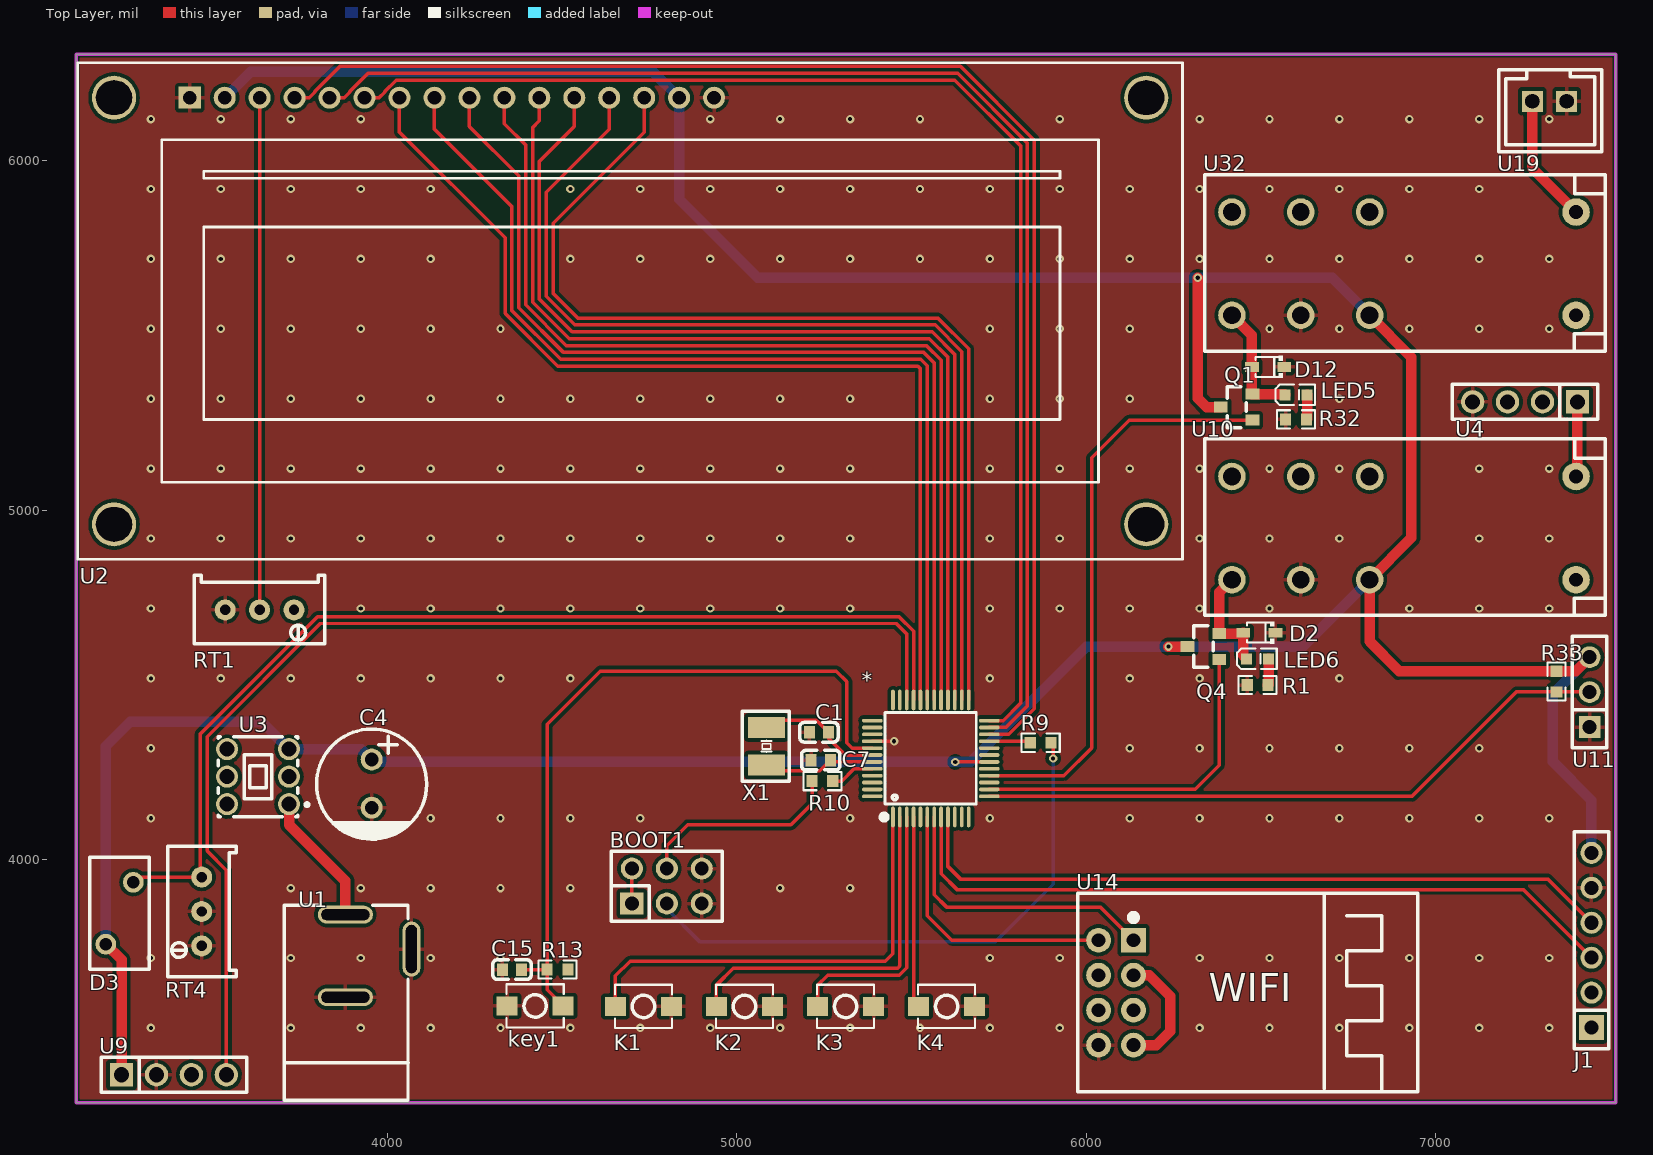
[diagram p0: Top Layer view]
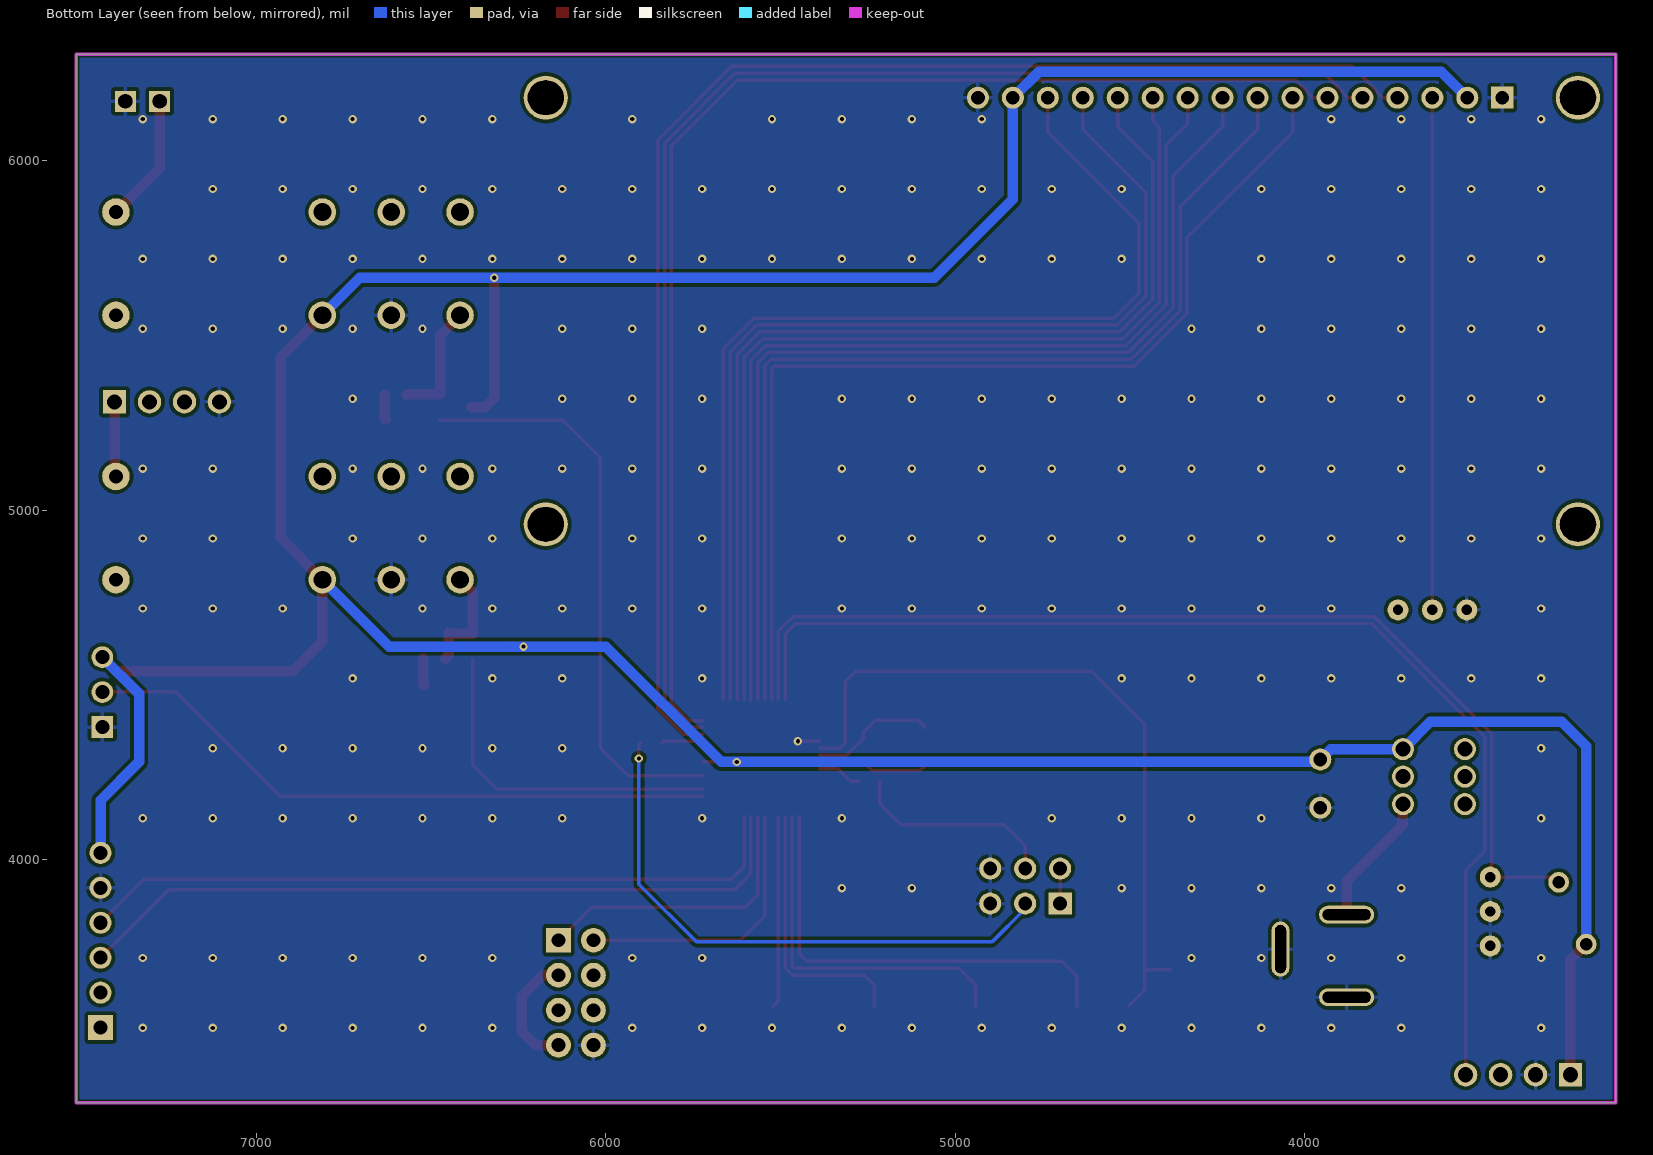
[diagram p1: Bottom Layer view, seen from below]
# Altium PCB MISC51945.pcbdoc
Units mil, origin at the board's own origin, x right, y up, seen from the top; angles counter-clockwise.
Board outline 4405 x 3000 mil, 2 copper layers (Top Layer, Bottom Layer), stack 62.206 mil thick; 38 components, 51 nets, 180 pads, 213 vias.

## Layer stack, top to bottom
Top Solder Mask Layer: solder mask 0.394, Dk 3.3
Top Layer: signal copper 1.379
Dielectric1: surface 59.449, FR4, Dk 4.5
Bottom Layer: signal copper 1.378
Bottom Solder Mask Layer: solder mask 0.394, Dk 3.3

## Board outline
3110,6305 3110,3305 7515,3305 7515,6305

## Design rules (kind name [scope] priority, off if disabled: settings)
BoardOutlineClearance copperThickness2oz_1 [All] p2 off: genericclearance=7.99 ignorepadtopadclearanceinfootprint=FALSE except(0: Arc-SplitContinuation Track-SplitContinuation SMDPad-SplitContinuation THPad-SplitContinuation Via-SplitContinuation Fill-SplitContinuation Region-SplitContinuation Poly-SplitContinuation Text-SplitContinuation Hole-SplitContinuation; 5.98: Arc-CutoutEdge SMDPad-CutoutEdge THPad-CutoutEdge Via-CutoutEdge Fill-CutoutEdge Region-CutoutEdge Text-CutoutEdge; 6.93: Hole-OutlineEdge Hole-CutoutEdge; 10: Poly-OutlineEdge Poly-CutoutEdge; 11.81: Arc-OutlineEdge Track-OutlineEdge SMDPad-OutlineEdge THPad-OutlineEdge Via-OutlineEdge Fill-OutlineEdge Region-OutlineEdge Text-OutlineEdge Track-CutoutEdge)
BoardOutlineClearance copperThickness1oz_1 [All] p4: genericclearance=4.02 ignorepadtopadclearanceinfootprint=FALSE except(0: Arc-SplitContinuation Track-SplitContinuation SMDPad-SplitContinuation THPad-SplitContinuation Via-SplitContinuation Fill-SplitContinuation Region-SplitContinuation Poly-SplitContinuation Text-SplitContinuation Hole-SplitContinuation; 6: SMDPad-CutoutEdge THPad-CutoutEdge Via-CutoutEdge Fill-CutoutEdge Region-CutoutEdge Text-CutoutEdge; 6.93: Hole-OutlineEdge Hole-CutoutEdge; 10: Poly-OutlineEdge Poly-CutoutEdge; 11.8: Arc-OutlineEdge Track-OutlineEdge SMDPad-OutlineEdge THPad-OutlineEdge Via-OutlineEdge Fill-OutlineEdge Region-OutlineEdge Text-OutlineEdge; 11.81: Arc-CutoutEdge Track-CutoutEdge)
Clearance copperThickness2oz [All] p1 off: gap=7.99 ignorepadtopadclearanceinfootprint=FALSE except(5.98: SMDPad-Track SMDPad-SMDPad THPad-Track SMDPad-THPad THPad-THPad Track-Via SMDPad-Via THPad-Via Via-Via Fill-Track Region-Track Fill-SMDPad Region-SMDPad Fill-THPad Region-THPad Fill-Via Region-Via Fill-Fill Fill-Region Region-Region Arc-Track Arc-SMDPad Arc-THPad Arc-Via Fill-Arc Region-Arc Arc-Arc Text-Track SMDPad-Text Text-THPad Text-Via Fill-Text Region-Text Arc-Text Text-Text; 6.93: Hole-Track Hole-SMDPad Hole-THPad Hole-Via Fill-Hole Region-Hole Hole-Arc Hole-Text; 10: Poly-Track Poly-SMDPad Poly-THPad Poly-Via Poly-Fill Poly-Region Poly-Poly Poly-Arc Poly-Text Poly-Hole)
Clearance copperThickness1oz [All] p3: gap=4.02 ignorepadtopadclearanceinfootprint=FALSE except(5.98: SMDPad-Track SMDPad-SMDPad THPad-Track SMDPad-THPad THPad-THPad Track-Via SMDPad-Via THPad-Via Via-Via Fill-Track Region-Track Fill-SMDPad Region-SMDPad Fill-THPad Region-THPad Fill-Via Region-Via Fill-Fill Fill-Region Region-Region; 6: Arc-Track Arc-SMDPad Arc-THPad Arc-Via Fill-Arc Region-Arc Arc-Arc Text-Track SMDPad-Text Text-THPad Text-Via Fill-Text Region-Text Arc-Text Text-Text; 6.93: Hole-Track Hole-SMDPad Hole-THPad Hole-Via Fill-Hole Region-Hole Hole-Arc Hole-Text; 10: Poly-Track Poly-SMDPad Poly-THPad Poly-Via Poly-Fill Poly-Region Poly-Poly Poly-Arc Poly-Text Poly-Hole)
DiffPairsRouting differentialPair [All] p1: maxlimit=6 minlimit=6 mostfreqgap=6 toplayer_minwidth=5 toplayer_prefwidth=10 toplayer_maxwidth=100 toplayer_mingap=6 toplayer_prefgap=6 toplayer_maxgap=6 bottomlayer_minwidth=5 bottomlayer_prefwidth=10 bottomlayer_maxwidth=100 bottomlayer_mingap=6 bottomlayer_prefgap=6 bottomlayer_maxgap=6 maxuncoupledlength=10
HoleToHoleClearance otherClearance [All] p1: gap=11.81 allowstackedmicrovias=TRUE
Length netLength [All] p1: minlimit=0 maxlimit=0
MatchedLengths netLengthTolerance [All] p1: tolerance=1000
PasteMaskExpansion pasteMaskExpansion [All] p1: expansion=0
PlaneConnect innerPlane [All] p1: planeconnectstyle=Relief reliefexpansion=20 reliefentries=4 reliefconductorwidth=10 reliefairgap=10
PolygonConnect copperRegion [(InNet('GND'))] p1: connectstyle=Relief reliefconductorwidth=10 reliefentries=4 polygonreliefangle="90 Angle" airgapwidth=10 via.connectstyle=Relief via.reliefconductorwidth=10 via.reliefentries=4 via.polygonreliefangle="90 Angle" via.airgapwidth=10
RoutingVias viaSize [All] p1: holewidth=12.01 width=24.02 viastyle="Through Hole" minholewidth=11.81 minwidth=19.68 maxholewidth=248.03 maxwidth=393.7
SolderMaskExpansion solderMaskExpansion [IsVia] p1: expansion=-1000 istentingtop=TRUE
SolderMaskExpansion solderMaskExpansion [All] p2: expansion=2 istentingtop=FALSE
Width copperThickness2oz_2 [All] p1 off: maxlimit=100 minlimit=8 preferedwidth=10
Width copperThickness1oz_2 [All] p2: maxlimit=100 minlimit=5 preferedwidth=10

## Components (designator, comment, footprint, x,y, rotation, side; value= is the part's Value field where it differs from the comment)
* "程序下载口" LQFP-48_L7.0-W7.0-P0.50-LS9.0-BL 5555,4290 r0 top
BOOT1 "Header 3X2" HDR-TH_6P-P2.54-V-F-R2-C3-S2.54 4800,3925 r0 top
C1 "20pF" C0603 5235,4365 r0 top
C4 "1000UF" CAP-TH_BD8.0-P3.50-D0.6-FD_1 3955.58,4218 r270 top
C7 "20pF" C0603 5240,4285 r0 top
C15 "104" C0603 4357.19,3686.05 r0 top
D2 "IN4148" SOD-323_L1.8-W1.3-LS2.5-RD 6495,4650 r180 top
D3 "光敏电阻" RES-TH_L8.0-W4.4-P4.50-D0.6-S2.0 3234.3,3847.2 r90 top
D12 "IN4148" SOD-323_L1.8-W1.3-LS2.5-RD 6520,5410 r180 top
J1 "" HDR-TH_6P-P2.54-V-F 7445,3770 r90 top
K1 "" Key_SMD_3x4x2 4733,3580.6 r180 top
K2 "" Key_SMD_3x4x2 5022.12,3580.6 r180 top
K3 "" Key_SMD_3x4x2 5311.24,3580.6 r180 top
K4 "" Key_SMD_3x4x2 5600.36,3580.6 r180 top
key1 "KEY_M" Key_SMD_3x4x2 4423.29,3582.1 r180 top
LED5 "LED" LED0603 6600,5330 r0 top
LED6 "LED" LED0603 6490,4575 r0 top
Q1 "S8050" S8050_SOT-23 6430,5295 r0 top
Q4 "S8050" S8050_SOT-23 6335,4610 r0 top
R1 "1K" R0603 6490,4500 r0 top
R9 "10K" R0603 5869.32,4335 r0 top
R10 "10K" R0603 5245,4225 r0 top
R13 "10 K" R0603 4487.19,3686.05 r180 top
R32 "1K" R0603 6600,5260 r0 top
R33 "10K" R0603 7344.9,4509.9 r90 top
RT1 "10K" R_3296 3635,4710 r180 top
RT4 "10K" R_3296 3464.3,3852.2 r90 top
U1 "POW" DC-2.0 3870,3720 r270 top
U2 "LCD1602" LCD1602 4695,5570 r0 top
U3 "SWITCH" SW-TH_6P-L5.8-W5.8-P2.00-LS4.5-TR 3630.58,4238 r270 top
U4 "" HDR-TH_4P-P2.54-V-F 7255,5310 r180 top
U9 "" HDR-TH_4P-P2.54-V-F 3390,3385 r0 top
U10 "JDQ-5" RELAY-TH_FTR-K1CK024W 6908.81,4948.98 r0 top
U11 "DHT11" HDR-TH_3P-P2.54-V-F 7439.9,4479.9 r90 top
U14 "ESP8266" WIFIM-TH_8P-L24.7-W14.4-P2.54 6085,3620 r0 top
U19 "" CONN-TH_XH2.54-2P 7325,6170 r180 top
U32 "JDQ-5" RELAY-TH_FTR-K1CK024W 6908.81,5705.51 r0 top
X1 "8MHz" CRYSTAL-SMD_L3.2-W2.5_3225-8MHZ 5085.08,4324.89 r90 top

## Footprints (in the part's own frame and the unit in brackets; to place one, negate y for a bottom-side part, rotate by r counter-clockwise, add the part's x,y. Pads: shape width x height; smd on the part's side, far side on the other; paste and mask are expansions set on the pad)
C0603 [mm]
  rect 0.8x0.9 smd: 1(-0.7,0) 2(0.7,0)
  silkscreen extent -1.39,-0.71 1.39,0.71
CAP-TH_BD8.0-P3.50-D0.6-FD_1 [mm]
  round 1.6 hole 1: 1(-1.75,0) 2(1.75,0)
  silkscreen extent -3.96,-4 4.04,4
CONN-TH_XH2.54-2P [mil]
  rect 60x60 hole 39.37 slot 41.34 at 0 deg paste+0 mask+1.97: 1(-49.22,0) 2(49.21,0)
  silkscreen extent -150,-90 145,145
CRYSTAL-SMD_L3.2-W2.5_3225-8MHZ [mil]
  rect 60x106.3 smd paste+0 mask+1.97: 1(-53.62,0) 2(53.62,0)
  silkscreen extent -100,-65 100,70
DC-2.0 [mil]
  oval 157.5x51.2 hole 31.5 slot 137.8 at 0 deg paste+0 mask+2: 2(-24.7,199.5)
  oval 51.2x157.5 hole 31.5 slot 137.8 at 90 deg paste+0 mask+2: 3(113.1,10.5) 4(-123.1,10.5)
  silkscreen extent -151,-165 408,190
HDR-TH_3P-P2.54-V-F [mil]
  rect 62x62 hole 40.16: 1(-100,0)
  round 62 hole 40.16: 2(0,0) 3(100,0)
  silkscreen extent -160,-49 160,49
HDR-TH_4P-P2.54-V-F [mm]
  rect 1.7x1.7 hole 1.1: 1(-3.81,0)
  round 1.7 hole 1.1: 2(-1.27,0) 3(1.27,0) 4(3.81,0)
  silkscreen extent -5.29,-1.27 5.29,1.27
HDR-TH_6P-P2.54-V-F [mm]
  rect 1.8x1.8 hole 1.02: 1(-6.35,0)
  round 1.6 hole 1.02: 2(-3.81,0) 3(-1.27,0) 4(1.27,0) 5(3.81,0) 6(6.35,0)
  silkscreen extent -7.87,-1.25 7.87,1.25
HDR-TH_6P-P2.54-V-F-R2-C3-S2.54 [mm]
  rect 1.7x1.6 hole 1: 1(-2.54,-1.27)
  round 1.6 hole 1: 2(-2.54,1.27) 3(0,-1.27) 4(0,1.27) 5(2.54,-1.27) 6(2.54,1.27)
  silkscreen extent -4.04,-2.54 4.04,2.54
Key_SMD_3x4x2 [mm]
  rect 1.53x1.36 smd paste+0 mask+0.051: 1(-2.035,0) 2(2.035,0)
  silkscreen extent -2.08,-1.58 2.08,1.58
LCD1602 [mm]
  round 3.2 hole 2.5 slot 2.625 at 0 deg: 0(-37.5,-15.5) 0(-37.5,15.5) 0(37.5,-15.5) 0(37.5,15.5)
  rect 1.6x1.6 hole 1: 1(-32,15.5)
  round 1.6 hole 1: 2(-29.46,15.5) 3(-26.92,15.5) 4(-24.38,15.5) 5(-21.84,15.5) 6(-19.3,15.5) 7(-16.76,15.5) 8(-14.22,15.5) 9(-11.68,15.5) 10(-9.14,15.5) 11(-6.6,15.5) 12(-4.06,15.5) 13(-1.52,15.5) 14(1.02,15.5) 15(3.56,15.5) 16(6.1,15.5)
  silkscreen extent -40.13,-18.03 40.13,18.03
LED0603 [mm]
  rect 0.8x0.8 smd: 1(-0.799,-0.003) 2(0.799,0.003)
  silkscreen extent -1.49,-0.75 1.39,0.76
LQFP-48_L7.0-W7.0-P0.50-LS9.0-BL [mm]
  oval 0.27x1.5 smd paste+0 mask+0.05: 1(-2.75,-4.25) 2(-2.25,-4.25) 3(-1.75,-4.25) 4(-1.25,-4.25) 5(-0.75,-4.25) 6(-0.25,-4.25) 7(0.25,-4.25) 8(0.75,-4.25) 9(1.25,-4.25) 10(1.75,-4.25) 11(2.25,-4.25) 12(2.75,-4.25) 25(2.75,4.25) 26(2.25,4.25) 27(1.75,4.25) 28(1.25,4.25) 29(0.75,4.25) 30(0.25,4.25) 31(-0.25,4.25) 32(-0.75,4.25) 33(-1.25,4.25) 34(-1.75,4.25) 35(-2.25,4.25) 36(-2.75,4.25)
  oval 1.5x0.27 smd paste+0 mask+0.05: 13(4.25,-2.75) 14(4.25,-2.25) 15(4.25,-1.75) 16(4.25,-1.25) 17(4.25,-0.75) 18(4.25,-0.25) 19(4.25,0.25) 20(4.25,0.75) 21(4.25,1.25) 22(4.25,1.75) 23(4.25,2.25) 24(4.25,2.75) 37(-4.25,2.75) 38(-4.25,2.25) 39(-4.25,1.75) 40(-4.25,1.25) 41(-4.25,0.75) 42(-4.25,0.25) 43(-4.25,-0.25) 44(-4.25,-0.75) 45(-4.25,-1.25) 46(-4.25,-1.75) 47(-4.25,-2.25) 48(-4.25,-2.75)
  silkscreen extent -3.59,-4.46 3.3,3.34
R0603 [mil]
  rect 31.75x34.02 smd paste-3937.01 mask+2: 1(-29.66,0) 2(29.66,0)
  silkscreen extent -55,-26 55,26
R_3296 [mil]
  round 60 hole 30 paste+0 mask+2: 1(-98.4,-5) 2(0,-5) 3(98.4,-5)
  silkscreen extent -187,-103 187,92
RELAY-TH_FTR-K1CK024W [mm]
  round 2 hole 1.3: 1(-12.5,-3.75) 2(-7.5,-3.75) 3(-2.5,-3.75) 6(-2.5,3.75) 7(-7.5,3.75) 8(-12.5,3.75)
  round 2 hole 1: 4(12.5,-3.75) 5(12.5,3.75)
  silkscreen extent -14.48,-6.35 14.6,6.48
RES-TH_L8.0-W4.4-P4.50-D0.6-S2.0 [mm]
  round 1.5 hole 0.9 paste+0 mask+0.05: 1(-2.25,1) 2(2.25,-1)
  silkscreen extent -4.06,-2.16 4.06,2.16
S8050_SOT-23 [mm]
  rect 1x0.8 smd paste+0 mask+0.051: 1(1.15,-0.95) 2(1.15,0.95) 3(-1.15,0)
  silkscreen extent -0.7,-1.5 0.7,1.5
SOD-323_L1.8-W1.3-LS2.5-RD [mm]
  rect 1x0.7 smd: 1(-1.172,0) 2(1.172,0)
  silkscreen extent -1.08,-0.8 0.9,0.8
SW-TH_6P-L5.8-W5.8-P2.00-LS4.5-TR [mm]
  round 1.6 hole 1.1: 1(2,2.25) 2(0,2.25) 3(-2,2.25) 4(-2,-2.25) 5(0,-2.25) 6(2,-2.25)
  silkscreen extent -2.9,-2.9 2.9,3.68
WIFIM-TH_8P-L24.7-W14.4-P2.54 [mm]
  rect 1.8x1.8 hole 1 paste+0 mask+0.05: 1(1.27,3.81)
  round 1.8 hole 1 paste+0 mask+0.05: 2(1.27,1.27) 3(1.27,-1.27) 4(1.27,-3.81) 5(-1.27,3.81) 6(-1.27,1.27) 7(-1.27,-1.27) 8(-1.27,-3.81)
  silkscreen extent -2.77,-7.19 21.93,7.24

## Via types
v1: diameter 24.02, hole 12, Top Layer to Bottom Layer, 213 vias

## Nets (pads, with @x,y where several pads share a name; then routed paths per layer and width w, separated by ;. In a path a pad name is that pad's centre, name@x,y a point inside that pad or via, vN(x,y) a via of type N, cw(c..) or ccw(c..) an arc to the next point about the centre after c; other vN are vias at no path point)
3.3V: R13.1
$2N44: *.20
$2N45: *.26 U2.13 | length 2893.2
  Top Layer w10: U2.13 4635.16,6089.82 4455.31,5909.97 4455.31,5611.84 4536.97,5530.18 5567.32,5530.18 5643.58,5453.92 *.26
$2N46: *.27 U2.12 | length 2859.9
  Top Layer w10: U2.12 4535.16,6097.97 4435.63,5998.44 4435.63,5603.69 4528.82,5510.5 5559.17,5510.5 5623.9,5445.77 *.27
$2N47: *.29 U2.10 | length 2844
  Top Layer w10: U2.10 4335.16,6106.13 4396.26,6045.03 4396.26,5587.38 4512.51,5471.13 5542.86,5471.13 5584.53,5429.46 *.29
$2N48: *.30 U2.9 | length 2877.3
  Top Layer w10: U2.9 4235.16,6097.97 4376.57,5956.56 4376.57,5579.23 4504.36,5451.44 5534.71,5451.44 5564.84,5421.31 *.30
$2N49: *.31 U2.8 | length 2910.5
  Top Layer w10: U2.8 4135.16,6089.82 4356.89,5868.09 4356.89,5571.08 4496.21,5431.76 5526.55,5431.76 5545.16,5413.16 *.31
$2N50: *.32 U2.7 | length 2943.8
  Top Layer w10: U2.7 4035.16,6081.67 4337.2,5779.63 4337.2,5562.92 4488.05,5412.07 5518.4,5412.07 5525.47,5405 *.32
$2N51: *.28 U2.11 | length 2826.6
  Top Layer w10: U2.11 4435.16,6114.28 4415.94,6095.06 4415.94,5595.54 4520.67,5490.81 5551.01,5490.81 5604.21,5437.62 *.28
$2N52: RT1.2 U2.3 | length 1465.3
  Top Layer w10: RT1.2 3635,6180.08 U2.3
$2N54: BOOT1.3 R9.2 | length 1635.2
  Top Layer w10: R9.2 5905,4328.98 v1(5905,4290)
  Bottom Layer w10: BOOT1.3 4800,3860 4895,3765 5740,3765 5905,3930 v1(5905,4290)
$2N55: BOOT1.4 R10.1 | length 594.8
  Top Layer w10: BOOT1.4 4800,4040 4860,4100 5155,4100 5215.34,4160.34 R10.1
$2N56: *.41 C15.2 key1.1 R13.2 | length 2084.4
  Top Layer w10: C15.2 R13.2 ; key1.1 4457.53,3627.97 R13.2 ; *.41 5330.47,4319.53 5315,4335 5315,4510 5285,4540 4610,4540 4457.53,4387.53 R13.2
$2N57: *.42 C1.2 X1.2 | length 363.3
  Top Layer w10: X1.2 5106.57,4400 5227.56,4400 C1.2 5262.56,4347.44 5310.16,4299.84 *.42
$2N58: U1.4 U3.1 | length 383
  Top Layer w30: U3.1 3719.16,4100.84 3880.5,3939.5 U1.4
$2N59: *.19
$2N60: D2.2 LED6.1 Q4.2 U10.1 | length 317.8
  Top Layer w30: U10.1 6380.28,4764.93 Q4.2 6446.24,4647.4 D2.2 6448.84,4584.55 LED6.1
$2N61: U19.2 U32.5 | length 368.7
  Top Layer w30: U19.2 7275.78,5978.3 U32.5
$2N62: D12.2 LED5.1 Q1.2 U32.1 | length 344
  Top Layer w30: U32.1 6473.84,5500.73 D12.2 6473.84,5333.84 Q1.2 6565.99,5332.4 LED5.1
$2N63: *.10
$2N64: *.25 U2.14 | length 2926.4
  Top Layer w10: U2.14 4735.16,6081.67 4475,5821.51 4475,5620 4545.13,5549.87 5575.48,5549.87 5663.27,5462.08 *.25
$2N65: *.24 U2.6 | length 3680.8
  Top Layer w10: U2.6 3976.66,6180.24 3992.68,6196.26 3992.68,6197.84 4025.47,6230.63 5623.69,6230.63 5811.79,6042.53 5811.79,4448.21 5761.85,4398.27 *.24
$2N66: *.23 U2.5 | length 3854.2
  Top Layer w10: U2.5 3876.66,6180.24 3892.68,6196.26 3892.68,6197.84 3945.16,6250.32 5631.85,6250.32 5831.48,6050.69 5831.48,4440.06 5770,4378.58 *.23
$2N67: *.22 U2.4 | length 4027.6
  Top Layer w10: U2.4 3776.66,6180.24 3792.68,6196.26 3792.68,6197.84 3864.84,6270 5640,6270 5851.16,6058.84 5851.16,4431.9 5778.16,4358.9 *.22
$2N69: *.5
$2N70: *.11
$2N71: *.12
$2N72: U4.1 U10.5 | length 215.1
  Top Layer w30: U10.5 7405,5100.68 U4.1
$2N73: *.15
$2N76: *.8 J1.3 | length 2122.3
  Top Layer w10: *.8 5584.53,3960.47 5630,3915 7250,3915 J1.3
$2N77: *.9 J1.4 | length 2049.3
  Top Layer w10: *.9 5604.21,3980.79 5640,3945 7320,3945 J1.4
$2N78: LED6.2 R1.2 | length 75.9
  Top Layer w30: R1.2 6521.48,4501.81 LED6.2
$2N79: LED5.2 R32.2 | length 70.9
  Top Layer w30: R32.2 6631.48,5261.81 LED5.2
+3V3: U14.2 U14.4 | length 351.4
  Top Layer w30: U14.4 6200,3470 6240,3510 6240,3610 6180,3670 U14.2
A9: *.6 U14.5 | length 801.6
  Top Layer w10: *.6 5545.16,3839.84 5615,3770 U14.5
A10: *.7 U14.1 | length 846.6
  Top Layer w10: *.7 5564.84,3900.16 5600,3865 6040,3865 U14.1
ADC1: *.34 U9.4 | length 3326.6
  Top Layer w10: U9.4 3540,3970 3484.69,4025.31 3484.69,4351.84 3808.92,4676.08 5456.08,4676.08 5486.1,4646.05 *.34
ADC2: *.33 D3.2 RT4.3 | length 3006.9
  Top Layer w10: D3.2 3288.49,3950.6 RT4.3 3465,3954.9 3465,4360 3800.77,4695.77 5464.23,4695.77 5505.79,4654.21 *.33
BOOT0: *.21 R9.1 | length 119.1
  Top Layer w10: *.21 5835.45,4339.21 R9.1
BOOT1: *.44 R10.2 | length 127.7
  Top Layer w10: R10.2 5300,4225 5335.47,4260.47 *.44
DS: *.13 R33.1 U11.2 | length 1841.4
  Top Layer w10: *.13 6931.73,4181.73 7230.24,4480.24 R33.1 7439.56,4480.24 U11.2
GND: *.40 BOOT1.5 BOOT1.6 C1.1 C4.2 C7.1 C15.1 D2.1 D12.1 J1.5 K1.1 K2.1 K3.1 K4.1 key1.2 R1.1 R32.1 RT1.3 RT4.1 RT4.2 U1.2 U1.3 U2.1 U2.16 U4.4 U9.2 U10.2 U11.1 U14.8 U19.1 U32.2 | length 62.3
  Top Layer w10: *.40 v1(5450,4339.21)
  other v1: 3324.1,3519.1 3724.1,3519.1 3924.1,3519.1 4124.1,3519.1 4324.1,3519.1 4524.1,3519.1 4724.1,3519.1 4924.1,3519.1 5124.1,3519.1 5324.1,3519.1 5524.1,3519.1 5724.1,3519.1 5924.1,3519.1 6324.1,3519.1 6524.1,3519.1 6724.1,3519.1 6924.1,3519.1 7124.1,3519.1 7324.1,3519.1 3324.1,3719.1 3724.1,3719.1 3924.1,3719.1 4124.1,3719.1 4324.1,3719.1 5724.1,3719.1 5924.1,3719.1 6324.1,3719.1 6524.1,3719.1 6724.1,3719.1 6924.1,3719.1 7124.1,3719.1 7324.1,3719.1 3724.1,3919.1 3924.1,3919.1 4124.1,3919.1 4324.1,3919.1 4524.1,3919.1 5124.1,3919.1 5324.1,3919.1 3324.1,4119.1 4124.1,4119.1 4324.1,4119.1 4524.1,4119.1 4724.1,4119.1 5324.1,4119.1 5724.1,4119.1 6124.1,4119.1 6324.1,4119.1 6524.1,4119.1 6724.1,4119.1 6924.1,4119.1 7124.1,4119.1 7324.1,4119.1 3324.1,4319.1 6124.1,4319.1 6324.1,4319.1 6524.1,4319.1 6724.1,4319.1 6924.1,4319.1 7124.1,4319.1 3324.1,4519.1 3524.1,4519.1 3724.1,4519.1 3924.1,4519.1 4124.1,4519.1 4324.1,4519.1 4524.1,4519.1 5724.1,4519.1 6124.1,4519.1 6324.1,4519.1 6724.1,4519.1 3324.1,4719.1 3924.1,4719.1 4124.1,4719.1 4324.1,4719.1 4524.1,4719.1 4724.1,4719.1 4924.1,4719.1 5124.1,4719.1 5324.1,4719.1 5724.1,4719.1 5924.1,4719.1 6124.1,4719.1 6324.1,4719.1 6524.1,4719.1 6924.1,4719.1 7124.1,4719.1 7324.1,4719.1 3324.1,4919.1 3524.1,4919.1 3724.1,4919.1 3924.1,4919.1 4124.1,4919.1 4324.1,4919.1 4524.1,4919.1 4724.1,4919.1 4924.1,4919.1 5124.1,4919.1 5324.1,4919.1 5724.1,4919.1 5924.1,4919.1 6324.1,4919.1 6524.1,4919.1 6724.1,4919.1 7124.1,4919.1 7324.1,4919.1 3324.1,5119.1 3524.1,5119.1 3724.1,5119.1 3924.1,5119.1 4124.1,5119.1 4324.1,5119.1 4524.1,5119.1 4724.1,5119.1 4924.1,5119.1 5124.1,5119.1 5324.1,5119.1 5724.1,5119.1 5924.1,5119.1 6124.1,5119.1 6324.1,5119.1 6524.1,5119.1 6724.1,5119.1 7124.1,5119.1 7324.1,5119.1 3324.1,5319.1 3524.1,5319.1 3724.1,5319.1 3924.1,5319.1 4124.1,5319.1 4324.1,5319.1 4524.1,5319.1 4724.1,5319.1 4924.1,5319.1 5124.1,5319.1 5324.1,5319.1 5724.1,5319.1 5924.1,5319.1 6124.1,5319.1 6724.1,5319.1 3324.1,5519.1 3524.1,5519.1 3724.1,5519.1 3924.1,5519.1 4124.1,5519.1 4324.1,5519.1 5724.1,5519.1 5924.1,5519.1 6124.1,5519.1 6524.1,5519.1 6724.1,5519.1 6924.1,5519.1 7124.1,5519.1 7324.1,5519.1 3324.1,5719.1 3524.1,5719.1 3724.1,5719.1 3924.1,5719.1 4124.1,5719.1 4524.1,5719.1 4724.1,5719.1 4924.1,5719.1 5124.1,5719.1 5324.1,5719.1 5524.1,5719.1 5724.1,5719.1 5924.1,5719.1 6124.1,5719.1 6324.1,5719.1 6524.1,5719.1 6724.1,5719.1 6924.1,5719.1 7124.1,5719.1 7324.1,5719.1 3324.1,5919.1 3524.1,5919.1 3724.1,5919.1 3924.1,5919.1 4124.1,5919.1 4524.1,5919.1 4724.1,5919.1 4924.1,5919.1 5124.1,5919.1 5324.1,5919.1 5524.1,5919.1 5724.1,5919.1 5924.1,5919.1 6124.1,5919.1 6324.1,5919.1 6524.1,5919.1 6724.1,5919.1 6924.1,5919.1 7124.1,5919.1 3324.1,6119.1 3524.1,6119.1 3724.1,6119.1 3924.1,6119.1 4924.1,6119.1 5124.1,6119.1 5324.1,6119.1 5524.1,6119.1 5924.1,6119.1 6324.1,6119.1 6524.1,6119.1 6724.1,6119.1 6924.1,6119.1 7124.1,6119.1 7324.1,6119.1
K1: *.1 K1.2 | length 1298.5
  Top Layer w10: K1.2 4652.88,3667.88 4695,3710 5425,3710 5446.73,3731.73 *.1
K2: *.2 K2.2 | length 1034.6
  Top Layer w10: K2.2 4942,3642 4990,3690 5460,3690 5466.42,3696.42 *.2
K3: *.3 K3.2 | length 767.8
  Top Layer w10: K3.2 5231.12,3641.12 5260,3670 5465,3670 5486.1,3691.1 *.3
K4: *.4 K4.2 | length 548.1
  Top Layer w10: *.4 5505.79,3595.06 K4.2
LED: *.16 Q1.1 | length 1660.3
  Top Layer w10: *.16 5935.79,4240.79 6015,4320 6015,5150 6122.6,5257.6 Q1.1
LED3: *.14 Q4.1 | length 988.8
  Top Layer w10: *.14 6311.42,4201.42 6380.28,4270.28 Q4.1
OSC_OUT: *.43 C7.2 X1.1 | length 323.8
  Top Layer w10: X1.1 5101.35,4255 5237.56,4255 C7.2 5272.4,4280.16 *.43
VCC: *.18 C4.1 D3.1 J1.6 Q1.3 Q4.3 R33.2 U2.2 U2.15 U3.3 U9.1 U10.3 U11.3 U32.3 | length 11567.1
  Top Layer w10: v1(5625,4280) 5722.16,4280 *.18
  Top Layer w30: D3.1 3240,3713.55 U9.1 ; v1(6235,4610) Q4.3 ; v1(6318.97,5665) 6318.97,5321.03 6345,5295 Q1.3 ; U32.3 6930,5438.27 6930,4920.96 U10.3 6810.39,4624.61 6895.44,4539.56 R33.2 7399.56,4539.56 U11.3
  Bottom Layer w30: D3.1 3194.93,4324.93 3265,4395 3640.9,4395 U3.3 3925.74,4316.74 C4.1 3962.48,4280 v1(5625,4280) 5670,4280 6000,4610 v1(6235,4610) 6619.04,4610 U10.3 ; U2.2 3609.92,6255 4760.4,6255 U2.15 4835.16,5889.84 5060,5665 v1(6318.97,5665) 6703.27,5665 U32.3 ; U11.3 7335,4475 7335,4280 7445,4170 J1.6
VCC_3.3V: BOOT1.1 BOOT1.2 | length 100
  Top Layer w10: BOOT1.1 BOOT1.2
pads on no net: *.17 *.35 *.36 *.37 *.38 *.39 *.45 *.46 *.47 *.48 J1.1 J1.2 RT1.1 U2.0 U3.2 U3.4 U3.5 U3.6 U4.2 U4.3 U9.3 U10.4 U10.6 U10.7 U10.8 U14.3 U14.6 U14.7 U32.4 U32.6 U32.7 U32.8

## Polygon pours and split planes (outlines as drawn)
GND on Top Layer (solid, remove dead copper, pour order 0): 3010,6420 3010,3000 7765,3000 7765,6420
GND on Bottom Layer (solid, remove dead copper, pour order 2): 3000,6390 3000,3040 7805,3040 7805,6390

## Keep-outs
Board Outline Layer:
  the board outline again, w10